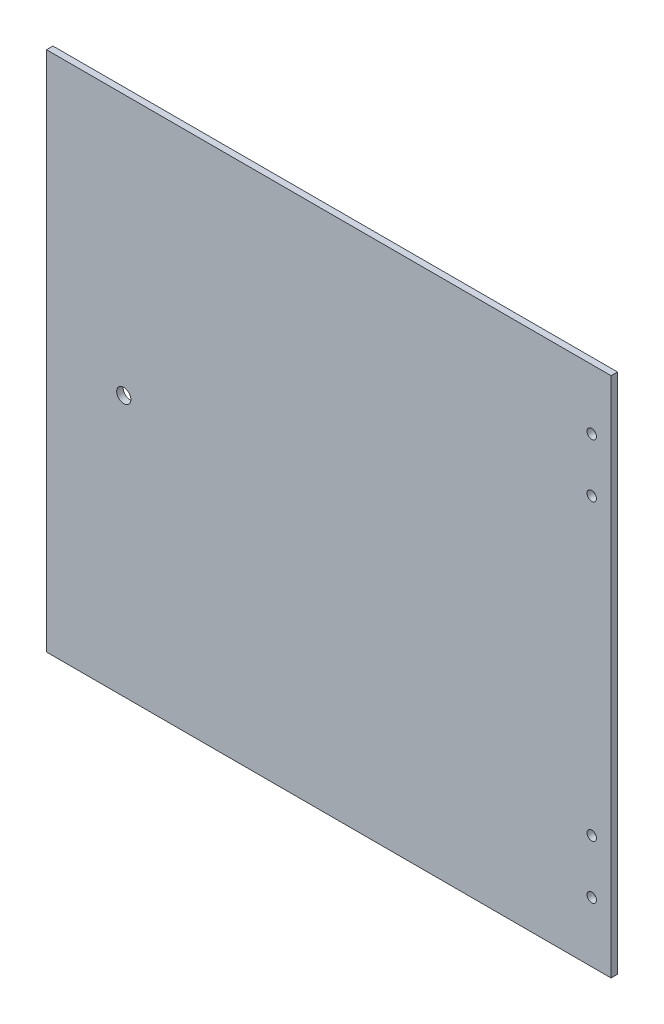
SolidWorks part; units mm, degrees
ref_plane "前视基准面" through (0, 0, 0) normal (0, 0, 1) x (1, 0, 0)
ref_plane "上视基准面" through (0, 0, 0) normal (0, 1, 0) x (1, 0, 0)
ref_plane "右视基准面" through (0, 0, 0) normal (1, 0, 0) x (0, 0, -1)
sketch "草图1" plane through (0, 0, 0) normal (0, 0, 1) x (1, 0, 0)
  line L1 (131.5, -121.5) -> (-131.5, -121.5)
  line L2 (131.5, -121.5) -> (131.5, 121.5)
  line L3 (131.5, 121.5) -> (-131.5, 121.5)
  line L4 (-131.5, -121.5) -> (-131.5, 121.5)
  line L5 (131.5, -121.5) -> (-131.5, 121.5) construction
  line L6 (131.5, 121.5) -> (-131.5, -121.5) construction
  point P0 (0, 0)
  dimension "D1" = 263
  dimension "D2" = 243
extrude "凸台-拉伸1" add sketch "草图1" along normal blind 3
sketch "草图4" plane through (0, 0, 0) normal (0, 0, -1) x (-1, 0, 0)
  line L0 (-122.5, -121.5) -> (-122.5, -93.5) construction
  line L1 (131.5, -121.5) -> (-131.5, -121.5) construction
  line L2 (-122.5, -93.5) -> (-122.5, -68.5) construction
  line L3 (-131.5, -121.5) -> (-131.5, 121.5) construction
  circle A0 centre (-122.5, -68.5) radius 2.2
  circle A1 centre (-122.5, -93.5) radius 2.2
  dimension "D1" = 4.4
  dimension "D2" = 25
  dimension "D3" = 28
  dimension "D4" = 9
extrude "切除-拉伸2" cut sketch "草图4" against normal blind 10
mirror "镜向1" about plane through (0, 0, 0) normal (0, 1, 0) of "切除-拉伸2"
sketch "草图5" plane through (0, 0, 3) normal (0, 0, 1) x (1, 0, 0)
  line L0 (-131.5, 0) -> (-95.5, 0) construction
  line L1 (-131.5, 121.5) -> (-131.5, -121.5) construction
  circle A0 centre (-95.5, 0) radius 3.3
  dimension "D2" = 6.6
  dimension "D1" = 36
extrude "切除-拉伸3" cut sketch "草图5" against normal blind 10
